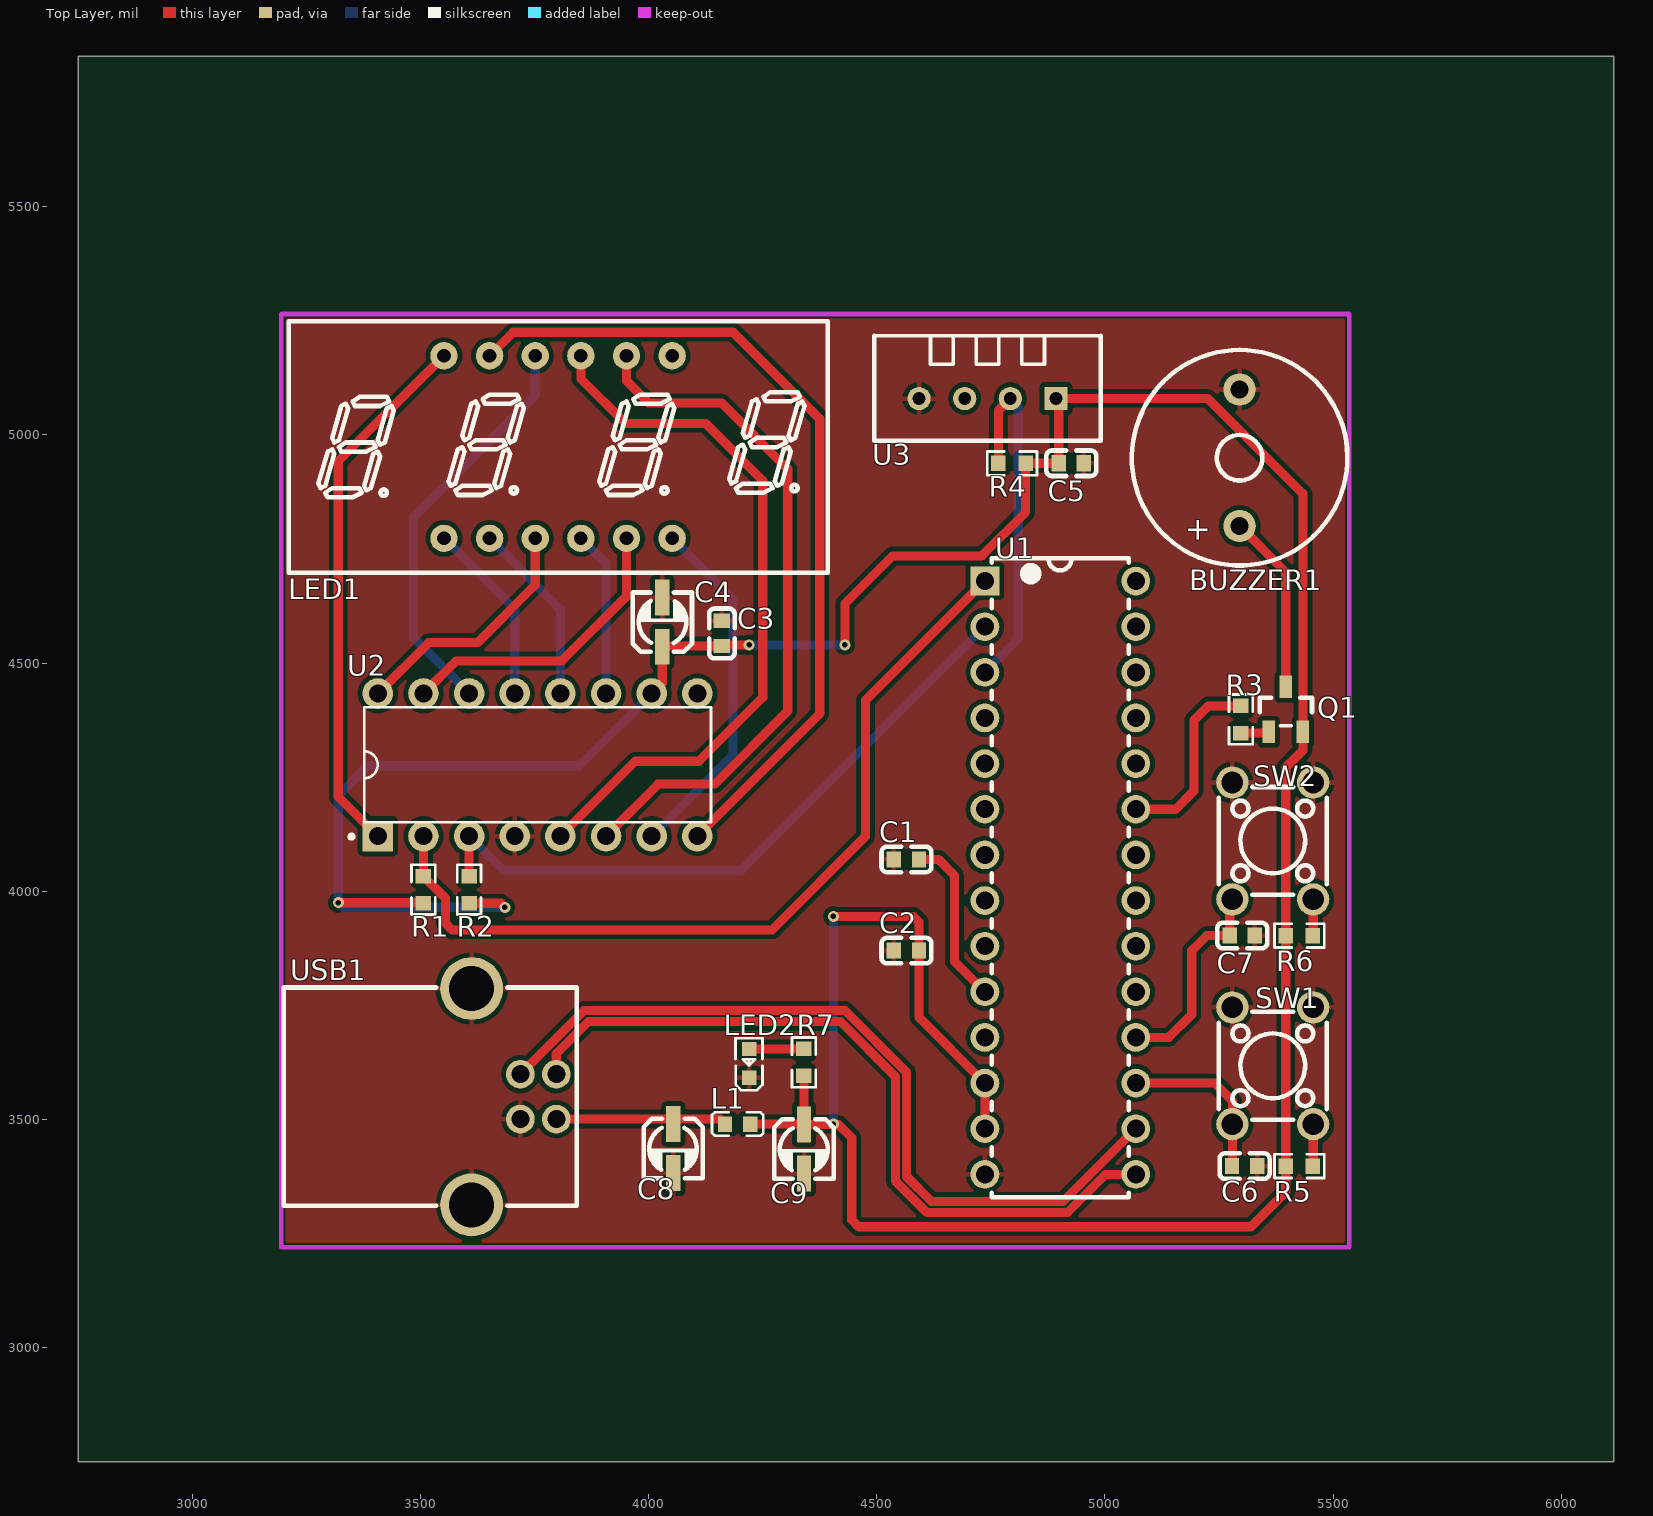
[diagram p0: Top Layer view]
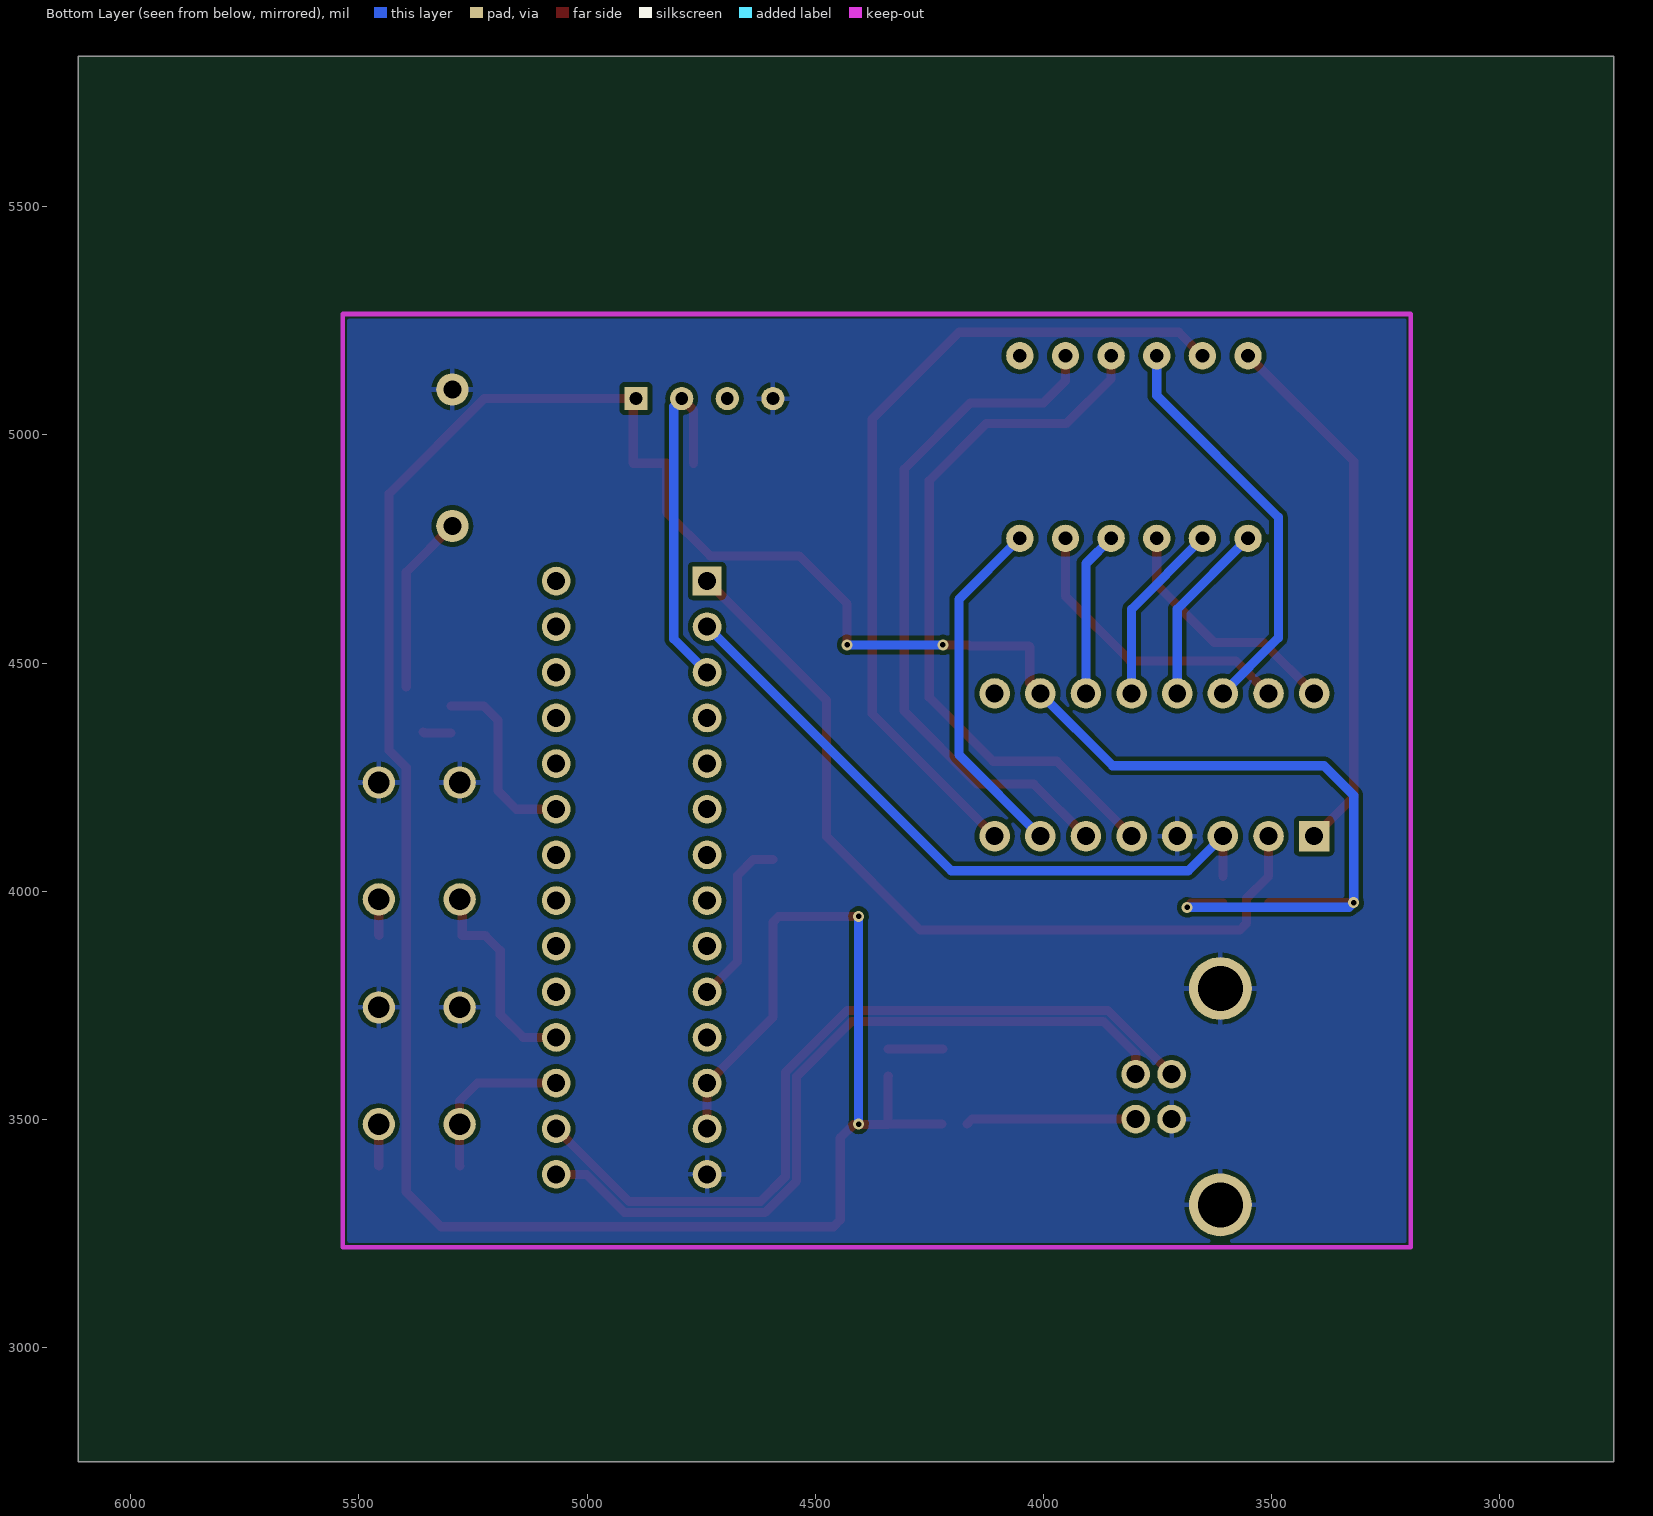
[diagram p1: Bottom Layer view, seen from below]
# Altium PCB MISC51906.pcbdoc
Units mil, origin at the board's own origin, x right, y up, seen from the top; angles counter-clockwise.
Board outline 3365 x 3080 mil, 2 copper layers (Top Layer, Bottom Layer), stack 62.206 mil thick; 27 components, 30 nets, 115 pads, 6 vias.

## Layer stack, top to bottom
Top Solder Mask Layer: solder mask 0.394, Dk 3.3
Top Layer: signal copper 1.379
Dielectric1: surface 59.449, FR4, Dk 4.5
Bottom Layer: signal copper 1.378
Bottom Solder Mask Layer: solder mask 0.394, Dk 3.3

## Board outline
6115,2750 2750,2750 2750,5830 6115,5830

## Design rules (kind name [scope] priority, off if disabled: settings)
BoardOutlineClearance copperThickness2oz_1 [All] p2 off: genericclearance=7.99 ignorepadtopadclearanceinfootprint=FALSE except(0: Arc-SplitContinuation Track-SplitContinuation SMDPad-SplitContinuation THPad-SplitContinuation Via-SplitContinuation Fill-SplitContinuation Region-SplitContinuation Poly-SplitContinuation Text-SplitContinuation Hole-SplitContinuation; 5.98: Arc-CutoutEdge SMDPad-CutoutEdge THPad-CutoutEdge Via-CutoutEdge Fill-CutoutEdge Region-CutoutEdge Text-CutoutEdge; 6.93: Hole-OutlineEdge Hole-CutoutEdge; 10: Poly-OutlineEdge Poly-CutoutEdge; 11.81: Arc-OutlineEdge Track-OutlineEdge SMDPad-OutlineEdge THPad-OutlineEdge Via-OutlineEdge Fill-OutlineEdge Region-OutlineEdge Text-OutlineEdge Track-CutoutEdge)
BoardOutlineClearance copperThickness1oz_1 [All] p4: genericclearance=4.02 ignorepadtopadclearanceinfootprint=FALSE except(0: Arc-SplitContinuation Track-SplitContinuation SMDPad-SplitContinuation THPad-SplitContinuation Via-SplitContinuation Fill-SplitContinuation Region-SplitContinuation Poly-SplitContinuation Text-SplitContinuation Hole-SplitContinuation; 6: SMDPad-CutoutEdge THPad-CutoutEdge Via-CutoutEdge Fill-CutoutEdge Region-CutoutEdge Text-CutoutEdge; 6.93: Hole-OutlineEdge Hole-CutoutEdge; 10: Poly-OutlineEdge Poly-CutoutEdge; 11.8: Arc-OutlineEdge Track-OutlineEdge SMDPad-OutlineEdge THPad-OutlineEdge Via-OutlineEdge Fill-OutlineEdge Region-OutlineEdge Text-OutlineEdge; 11.81: Arc-CutoutEdge Track-CutoutEdge)
Clearance copperThickness2oz [All] p1 off: gap=7.99 ignorepadtopadclearanceinfootprint=FALSE except(5.98: SMDPad-Track SMDPad-SMDPad THPad-Track SMDPad-THPad THPad-THPad Track-Via SMDPad-Via THPad-Via Via-Via Fill-Track Region-Track Fill-SMDPad Region-SMDPad Fill-THPad Region-THPad Fill-Via Region-Via Fill-Fill Fill-Region Region-Region Arc-Track Arc-SMDPad Arc-THPad Arc-Via Fill-Arc Region-Arc Arc-Arc Text-Track SMDPad-Text Text-THPad Text-Via Fill-Text Region-Text Arc-Text Text-Text; 6.93: Hole-Track Hole-SMDPad Hole-THPad Hole-Via Fill-Hole Region-Hole Hole-Arc Hole-Text; 10: Poly-Track Poly-SMDPad Poly-THPad Poly-Via Poly-Fill Poly-Region Poly-Poly Poly-Arc Poly-Text Poly-Hole)
Clearance copperThickness1oz [All] p3: gap=4.02 ignorepadtopadclearanceinfootprint=FALSE except(5.98: SMDPad-Track SMDPad-SMDPad THPad-Track SMDPad-THPad THPad-THPad Track-Via SMDPad-Via THPad-Via Via-Via Fill-Track Region-Track Fill-SMDPad Region-SMDPad Fill-THPad Region-THPad Fill-Via Region-Via Fill-Fill Fill-Region Region-Region; 6: Arc-Track Arc-SMDPad Arc-THPad Arc-Via Fill-Arc Region-Arc Arc-Arc Text-Track SMDPad-Text Text-THPad Text-Via Fill-Text Region-Text Arc-Text Text-Text; 6.93: Hole-Track Hole-SMDPad Hole-THPad Hole-Via Fill-Hole Region-Hole Hole-Arc Hole-Text; 10: Poly-Track Poly-SMDPad Poly-THPad Poly-Via Poly-Fill Poly-Region Poly-Poly Poly-Arc Poly-Text Poly-Hole)
DiffPairsRouting differentialPair [All] p1: maxlimit=6 minlimit=6 mostfreqgap=6 toplayer_minwidth=5 toplayer_prefwidth=10 toplayer_maxwidth=100 toplayer_mingap=6 toplayer_prefgap=6 toplayer_maxgap=6 bottomlayer_minwidth=5 bottomlayer_prefwidth=10 bottomlayer_maxwidth=100 bottomlayer_mingap=6 bottomlayer_prefgap=6 bottomlayer_maxgap=6 maxuncoupledlength=10
HoleToHoleClearance otherClearance [All] p1: gap=11.81 allowstackedmicrovias=TRUE
Length netLength [All] p1: minlimit=0 maxlimit=0
MatchedLengths netLengthTolerance [All] p1: tolerance=1000
PasteMaskExpansion pasteMaskExpansion [All] p1: expansion=0
PlaneConnect innerPlane [All] p1: planeconnectstyle=Relief reliefexpansion=20 reliefentries=4 reliefconductorwidth=10 reliefairgap=10
PolygonConnect copperRegion [(InNet('GND'))] p1: connectstyle=Relief reliefconductorwidth=10 reliefentries=4 polygonreliefangle="90 Angle" airgapwidth=10 via.connectstyle=Relief via.reliefconductorwidth=10 via.reliefentries=4 via.polygonreliefangle="90 Angle" via.airgapwidth=10
RoutingVias viaSize [All] p1: holewidth=12.01 width=24.02 viastyle="Through Hole" minholewidth=11.81 minwidth=19.68 maxholewidth=248.03 maxwidth=393.7
SolderMaskExpansion solderMaskExpansion [IsVia] p1: expansion=-1000 istentingtop=TRUE
SolderMaskExpansion solderMaskExpansion [All] p2: expansion=2 istentingtop=FALSE
Width copperThickness2oz_2 [All] p1 off: maxlimit=100 minlimit=8 preferedwidth=10
Width copperThickness1oz_2 [All] p2: maxlimit=100 minlimit=5 preferedwidth=10

## Components (designator, comment, footprint, x,y, rotation, side; value= is the part's Value field where it differs from the comment)
BUZZER1 "2.4kHz" BUZ-TH_BD12.0-P7.60-D0.6-FD 5295,4950 r90 top
C1 "1uF" C0603 4565.03,4069.86 r0 top
C2 "100nF" C0603 4565,3870 r0 top
C3 "100nF" C0603 4160.43,4564.97 r270 top
C4 "10uF" C_Ele_SMD_3x5.4mm 4030.43,4589.97 r270 top
C5 "100nF" C0603 4926.3,4937.94 r180 top
C6 "100nF" C0603 5305.85,3398.03 r180 top
C7 "100nF" C0603 5300.85,3903.03 r180 top
C8 "10uF" C_Ele_SMD_3x5.4mm 4053.58,3436.05 r90 top
C9 "10uF" C_Ele_SMD_3x5.4mm 4340,3435 r90 top
L1 "10uH" L0603 4195,3490 r0 top
LED1 "FJ3461AH" LED-SEG-TH_12P-L30.0-W14.0-P2.54-S10.16-BL 3801.53,4973.47 r0 top
LED2 "" LED_0603 4220,3625 r90 top
Q1 "" S8550P_SOT 5396.17,4400.21 r270 top
R1 "10K" R0603 3506.53,4003.47 r270 top
R2 "10K" R0603 3606.53,4003.47 r270 top
R3 "2K" R0603 5297.99,4376.51 r270 top
R4 "10K" R0603 4796.3,4937.94 r0 top
R5 "10K" R0603 5425.85,3398.03 r180 top
R6 "10K" R0603 5425.85,3903.03 r180 top
R7 "10K" R0603 4340,3625 r270 top
SW1 "" SW-TH_4P-L6.0-W6.0-P4.50-LS6.5 5367.68,3617.66 r90 top
SW2 "" SW-TH_4P-L6.0-W6.0-P4.50-LS6.5 5367.68,4110.43 r90 top
U1 "STC8H8K64U-45I-SKDIP28" DIP-28_L35.3-W7.3-P2.54-LS8.4-BL 4902.17,4029.86 r270 top
U2 "TM1650-DIP16" DIP-16_L19.3-W6.4-P2.54-LS8.0-BL 3756.67,4277.24 r0 top
U3 "DHT11" SENSOR-TH_DHT11 4742.54,5079.77 r180 top
USB1 "USB-B10-BRW" USB-B-TH_USB-B10-BRW 3705,3550 r270 top

## Footprints (in the part's own frame and the unit in brackets; to place one, negate y for a bottom-side part, rotate by r counter-clockwise, add the part's x,y. Pads: shape width x height; smd on the part's side, far side on the other; paste and mask are expansions set on the pad)
BUZ-TH_BD12.0-P7.60-D0.6-FD [mm]
  round 1.8 hole 1: 1(-3.8,0) 2(3.8,0)
  silkscreen extent -6,-6 6,6
C0603 [mm]
  rect 0.8x0.9 smd: 1(-0.7,0) 2(0.7,0)
  silkscreen extent -1.39,-0.71 1.39,0.71
C_Ele_SMD_3x5.4mm [mil]
  rect 78.7x31.5 smd paste+0 mask+2: 1(54.1,-0.55) 2(-53.7,-0.55)
  silkscreen extent -65,-65 65,65
DIP-16_L19.3-W6.4-P2.54-LS8.0-BL [mm]
  rect 1.7x1.7 hole 1: 1(-8.89,-3.97)
  round 1.7 hole 1: 2(-6.35,-3.97) 3(-3.81,-3.97) 4(-1.27,-3.97) 5(1.27,-3.97) 6(3.81,-3.97) 7(6.35,-3.97) 8(8.89,-3.97) 9(8.89,3.97) 10(6.35,3.97) 11(3.81,3.97) 12(1.27,3.97) 13(-1.27,3.97) 14(-3.81,3.97) 15(-6.35,3.97) 16(-8.89,3.97)
  silkscreen extent -10.46,-4.1 9.65,3.2
DIP-28_L35.3-W7.3-P2.54-LS8.4-BL [mm]
  rect 1.6x1.6 hole 1: 1(-16.51,-4.2)
  round 1.6 hole 1: 2(-13.97,-4.2) 3(-11.43,-4.2) 4(-8.89,-4.2) 5(-6.35,-4.2) 6(-3.81,-4.2) 7(-1.27,-4.2) 8(1.27,-4.2) 9(3.81,-4.2) 10(6.35,-4.2) 11(8.89,-4.2) 12(11.43,-4.2) 13(13.97,-4.2) 14(16.51,-4.2) 15(16.51,4.2) 16(13.97,4.2) 17(11.43,4.2) 18(8.89,4.2) 19(6.35,4.2) 20(3.81,4.2) 21(1.27,4.2) 22(-1.27,4.2) 23(-3.81,4.2) 24(-6.35,4.2) 25(-8.89,4.2) 26(-11.43,4.2) 27(-13.97,4.2) 28(-16.51,4.2)
  silkscreen extent -17.78,-3.81 17.78,3.81
L0603 [mm]
  rect 0.8x0.864 smd paste-100 mask+0.051: 1(-0.7,0) 2(0.7,0)
  silkscreen extent -1.42,-0.65 1.42,0.65
LED-SEG-TH_12P-L30.0-W14.0-P2.54-S10.16-BL [mil]
  round 60 hole 30: 1(-250,-200) 2(-150,-200) 3(-50,-200) 4(50,-200) 5(150,-200) 6(250,-200) 7(250,200) 8(150,200) 9(50,200) 10(-50,200) 11(-150,200) 12(-250,200)
  silkscreen extent -591,-276 591,276
LED_0603 [mil]
  rect 31.5x31.5 smd paste+0 mask+2: 1(-33.5,-0.4) 2(29.5,-0.2)
  silkscreen extent -61,-30 53,30
R0603 [mil]
  rect 31.75x34.02 smd paste-3937.01 mask+2: 1(-29.66,0) 2(29.66,0)
  silkscreen extent -55,-26 55,26
S8550P_SOT [mil]
  rect 49.2x27.6 smd paste+0 mask+2: 1(50.84,-37.4) 2(50.84,37.4) 3(-47.56,0)
  silkscreen extent -24,-58 37,58
SENSOR-TH_DHT11 [mil]
  rect 51x51 hole 28: 1(-150,0)
  round 51 hole 28: 2(-50,0) 3(50,0) 4(150,0)
  silkscreen extent -248,-138 248,93
SW-TH_4P-L6.0-W6.0-P4.50-LS6.5 [mm]
  round 1.8 hole 1.2: 1(-3.25,2.25) 2(3.25,2.25) 3(-3.25,-2.25) 4(3.25,-2.25)
  silkscreen extent -3,-3 3,3
USB-B-TH_USB-B10-BRW [mm]
  round 1.6 hole 1: 1(1.25,2.355) 2(-1.25,2.355) 3(-1.25,0.355) 4(1.25,0.355)
  round 3.5 hole 2.5: 5(-6.02,-2.355) 6(6.02,-2.355)
  silkscreen extent -6.08,-12.81 6.07,3.49

## Via types
v1: diameter 24.02, hole 12, Top Layer to Bottom Layer, 6 vias

## Nets (pads, with @x,y where several pads share a name; then routed paths per layer and width w, separated by ;. In a path a pad name is that pad's centre, name@x,y a point inside that pad or via, vN(x,y) a via of type N, cw(c..) or ccw(c..) an arc to the next point about the centre after c; other vN are vias at no path point)
$1N4: C1.2 U1.10 | length 374.7
  Top Layer w20: C1.2 4635.14,4069.86 4670,4035 4670,3846.68 U1.10
$1N54: Q1.1 R3.2 | length 61.8
  Top Layer w20: R3.2 5356.24,4346.85 Q1.1
$1N56: BUZZER1.1 Q1.3 | length 394.5
  Top Layer w20: BUZZER1.1 5396.17,4699.23 Q1.3
$1N63: R5.1 SW1.3 | length 92
  Top Layer w20: R5.1 5456.26,3398.78 SW1.3
$1N70: R6.1 SW2.3 | length 79.8
  Top Layer w20: R6.1 5456.26,3903.78 SW2.3
$1N77: LED2.2 R7.1 | length 119.9
  Top Layer w20: LED2.2 4339.84,3654.5 R7.1
+5V: C2.2 C3.2 C4.1 C5.2 C9.1 L1.2 Q1.2 R1.2 R2.2 R4.2 R5.2 R6.2 R7.2 U1.12 U1.13 U2.10 U3.1 | length 7903.1
  Top Layer w20: v1(3320,3975) 3505.34,3975 R1.2 ; R2.2 3676.19,3973.81 v1(3685,3965) ; U2.10 4029.88,4456.74 C4.1 4031.42,4537.41 C3.2 4163.01,4540 v1(4220,4540) ; L1.2 4339.65,3490 C9.1 ; R7.2 4340.55,3594.79 C9.1 ; v1(4405,3945) 4580,3945 4592.56,3932.44 C2.2 4592.56,3724.12 U1.12 U1.13 ; v1(4430,4540) 4430,4630 4535,4735 4730,4735 4825.96,4830.96 R4.2 C5.2 4898.74,5073.56 U3.1 5225.23,5079.77 5433.57,4871.43 Q1.2 5433.57,4308.57 5396.19,4271.19 R6.2 R5.2 5396.19,3341.19 5320,3265 4460,3265 4445,3280 4445,3460 4415.9,3489.1 C9.1
  Bottom Layer w20: v1(3685,3965) 3330,3965 v1(3320,3975) 3320,4210 3385,4275 3848.13,4275 U2.10 ; v1(4220,4540) v1(4430,4540) ; v1(4405,3490) v1(4405,3945)
A/K1: LED1.11 U2.8 | length 1848.7
  Top Layer w20: LED1.11 3703.06,5225 4185,5225 4375,5035 4375,4389.27 U2.8
B/K2: U2.9
BUZZ: R3.1 U1.23 | length 415
  Top Layer w20: U1.23 5154.86,4179.86 5195,4220 5195,4375 5226.17,4406.17 R3.1
C/K3: LED1.4 U2.11 | length 362.8
  Bottom Layer w20: LED1.4 3906.67,4718.33 U2.11
D/K4: LED1.2 U2.12 | length 404.2
  Bottom Layer w20: LED1.2 3806.67,4618.33 U2.12
DIG1: LED1.12 U2.1 | length 1184.3
  Top Layer w20: U2.1 3320,4207.61 3320,4941.94 LED1.12
DIG2: LED1.9 U2.5 | length 1585.3
  Top Layer w20: U2.5 3970.73,4285 4110,4285 4250,4425 4250,4900 4125,5025 3950,5025 3851.53,5123.47 LED1.9
DIG3: LED1.8 U2.6 | length 1530.5
  Top Layer w20: U2.6 4020.73,4235 4145,4235 4305,4395 4305,4925 4160,5070 4000,5070 3951.53,5118.47 LED1.8
DIG4: LED1.6 U2.7 | length 781.7
  Bottom Layer w20: U2.7 4185,4299.27 4185,4640 LED1.6
DIS_CLK: R1.1 U1.1 U2.2 | length 1890.5
  Top Layer w20: U2.2 3506.67,4033.27 R1.1 3555,3984.66 3555,3930 3570,3915 4270,3915 4475,4120 4475,4418.03 U1.1
DIS_DAT: R2.1 U1.2 U2.3 | length 1471
  Top Layer w20: R2.1 3606.67,4033.27 U2.3
  Bottom Layer w20: U2.3 3682.61,4045 4201.97,4045 U1.2
DP/KP: LED1.3 U2.16 | length 545.4
  Top Layer w20: U2.16 3518.13,4545 3625,4545 3751.53,4671.53 LED1.3
E/K5: LED1.1 U2.13 | length 404.2
  Bottom Layer w20: LED1.1 3706.67,4618.33 U2.13
F/K6: LED1.10 U2.14 | length 900.7
  Bottom Layer w20: U2.14 3485,4555.21 3485,4820 3751.53,5086.53 LED1.10
G/K7: LED1.5 U2.15 | length 660
  Top Layer w20: U2.15 3578.13,4505 3810,4505 3951.53,4646.53 LED1.5
GND: BUZZER1.2 C1.1 C2.1 C3.1 C4.2 C5.1 C6.1 C7.1 C8.2 C9.2 LED2.1 SW1.2 SW1.4 SW2.2 SW2.4 U1.14 U2.4 U3.4 USB1.4 USB1.5 USB1.6
KEY1: C6.2 SW1.1 U1.17 | length 370.9
  Top Layer w20: U1.17 5240.14,3579.86 5279.1,3540.9 SW1.1 5279.1,3398.84 C6.2
KEY2: C7.2 SW2.1 U1.18 | length 462.1
  Top Layer w20: U1.18 5139.86,3679.86 5190,3730 5190,3870 5223.03,3903.03 C7.2 5273.29,3976.67 SW2.1
NET24: LED1.7
SEN_DAT: R4.1 U1.3 U3.2 | length 790
  Top Layer w20: R4.1 4766.64,5053.88 U3.2
  Bottom Layer w20: U1.3 4810,4553.03 4810,5062.31 U3.2
USB_D+: U1.16 USB1.3 | length 1780.4
  Top Layer w20: USB1.3 3858.78,3739.02 4429.95,3739.02 4565,3603.96 4565,3375 4620,3320 4907.67,3320 U1.16
USB_D-: U1.15 USB1.2 | length 1686.4
  Top Layer w20: USB1.2 3797.72,3643.99 3868.72,3715 4420,3715 4540.98,3594.02 4540.98,3365.05 4610.05,3295.98 4917.61,3295.98 5001.49,3379.86 U1.15
VBUS: C8.1 L1.1 USB1.1 | length 374.2
  Top Layer w20: USB1.1 4156.66,3500.78 L1.1
pads on no net: U1.4 U1.5 U1.6 U1.7 U1.8 U1.9 U1.11 U1.19 U1.20 U1.21 U1.22 U1.24 U1.25 U1.26 U1.27 U1.28 U3.3

## Polygon pours and split planes (outlines as drawn)
GND on Top Layer (solid, remove dead copper, pour order 0): 3000,5580 3000,3000 5865,3000 5865,5580
GND on Bottom Layer (solid, remove dead copper, pour order 2): 3090,5450 3090,3135 5830,3135 5830,5450

## Keep-outs
Board Outline Layer:
  lines w10: 3195,3220 3195,5265 5535,5265 5535,3220 3195,3220